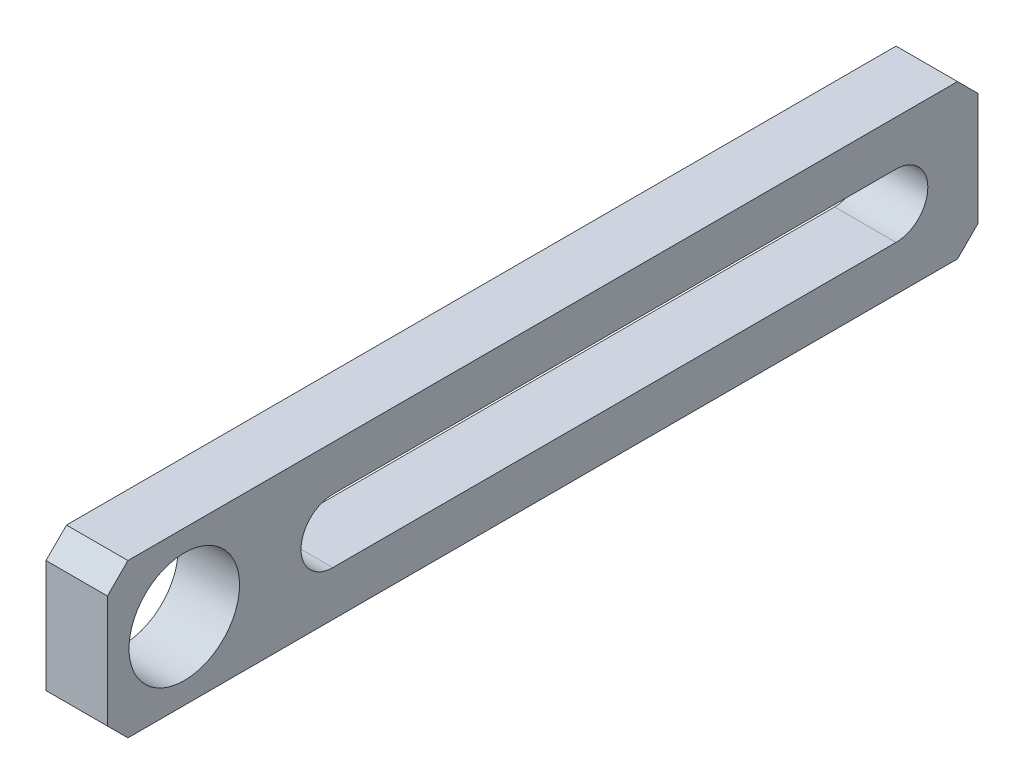
SolidWorks part; units mm, degrees
material "6061-T6"
ref_plane "Front Plane" through (0, 0, 0) normal (0, 0, 1) x (1, 0, 0)
ref_plane "Top Plane" through (0, 0, 0) normal (0, 1, 0) x (1, 0, 0)
ref_plane "Right Plane" through (0, 0, 0) normal (1, 0, 0) x (0, 0, -1)
sketch "Sketch1" plane through (0, 0, 0) normal (1, 0, 0) x (0, 0, -1)
  line L0 (22, -4.4) -> (77, -4.4)
  line L1 (0, 0) -> (85, 0)
  line L2 (0, 0) -> (0, -15)
  line L3 (0, -15) -> (85, -15)
  line L4 (85, 0) -> (85, -15)
  line L5 (22, -10.6) -> (77, -10.6)
  arc A0 (77, -10.6) -> (77, -4.4) centre (77, -7.5) ccw
  arc A1 (22, -4.4) -> (22, -10.6) centre (22, -7.5) ccw
  dimension "D6" = 6.2
  dimension "D1" = 85
  dimension "D2" = 15
  dimension "D3" = 8
  dimension "D4" = 7.5
  dimension "D5" = 55
extrude "Extrude1" add sketch "Sketch1" along normal blind 6
hole_wizard "M12x1.0 Tapped Hole1" positions "Sketch4" profile "Sketch3" tap size "M12x1.25" standard "ISO" end condition through all
sketch "Sketch4" plane through (6, 0, 0) normal (1, 0, 0) x (0, 0, -1)
  line L1 (0, -15) -> (85, -15) construction
  line L2 (0, 0) -> (0, -15) construction
  point P0 (7.5, -7.5)
  dimension "D1" = 7.5
  dimension "D2" = 7.5
sketch "Sketch3" plane through (6, -7.5, -7.5) normal (0, 1, 0) x (0, 0, -1)
  line L0 (0, 0) -> (0, 6)
  line L1 (0, 6) -> (5.4, 6)
  line L2 (5.4, 6) -> (5.4, 0)
  line L5 (5.4, 0) -> (0, 0)
  line L11 (0, -6.35) -> (0, 107.95) construction
  dimension "籵謂蹟恇謂郰芛眻噤" = 10.8
  dimension "籵謂蹟恇謂郰芛旮僅" = 6
cosmetic thread "Cosmetic thread1" parameters "D2"=12
chamfer "Chamfer1" distance 2 angle 45 4 edges at (3, 0, -85) (3, -15, -85) (3, -15, 0) (3, 0, 0)
